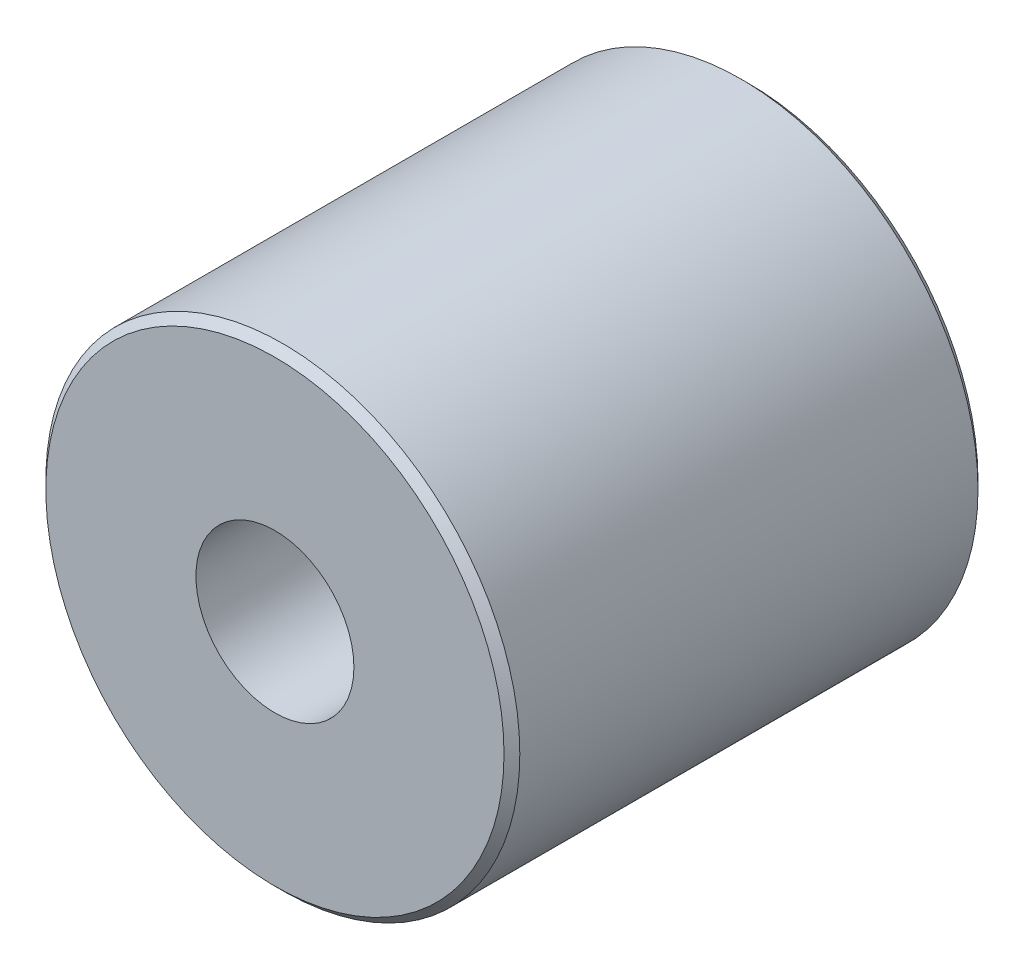
from build123d import *

# Parameters (mm, degrees)
SKETCH1_R           = 15
SKETCH1_R_2         = 5
BOSS_EXTRUDE1_DEPTH = 30
CHAMFER1_SIZE       = 0.5


with BuildPart() as part:
    # Sketch1 → Boss-Extrude1 (new body)
    with BuildSketch(Plane.XY):
        Circle(SKETCH1_R)
        Circle(SKETCH1_R_2, mode=Mode.SUBTRACT)
    extrude(amount=BOSS_EXTRUDE1_DEPTH)

    # Chamfer1
    chamfer1_edges = [part.edges().sort_by_distance(p)[0] for p in [
        (-15, 0, 0),
        (-15, 0, 30),
    ]]
    chamfer(chamfer1_edges, length=CHAMFER1_SIZE)


solid = part.part
